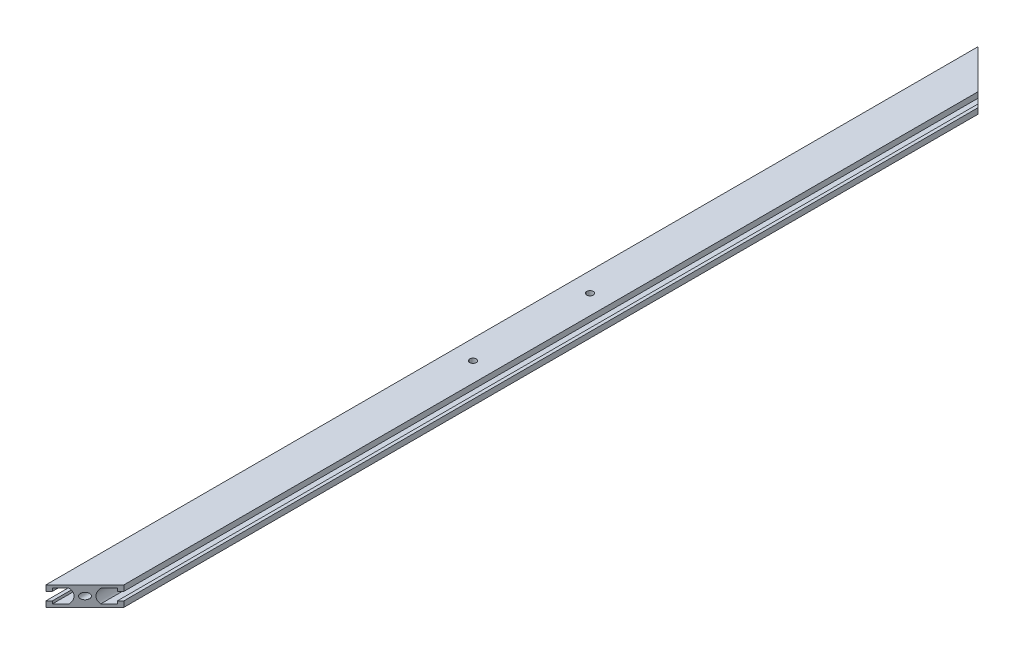
SolidWorks part; units mm, degrees
material "铝型材"
ref_plane "前视基准面" through (0, 0, 0) normal (0, 0, 1) x (1, 0, 0)
ref_plane "上视基准面" through (0, 0, 0) normal (0, 1, 0) x (1, 0, 0)
ref_plane "右视基准面" through (0, 0, 0) normal (1, 0, 0) x (0, 0, -1)
sketch "Model" plane through (0, 0, 0) normal (0, 0, 1) x (1, 0, 0)
  line L0 (2390.4271, 419.7568) -> (2392.9271, 419.7568)
  line L1 (2390.4271, 419.7568) -> (2390.4271, 417.7068)
  line L2 (2392.9271, 415.4068) -> (2392.9271, 419.7568)
  line L3 (2383.9948, 417.7068) -> (2390.4271, 417.7068)
  line L4 (2362.9271, 415.4068) -> (2392.9271, 415.4068)
  line L5 (2362.9271, 415.4068) -> (2362.9271, 419.7568)
  line L6 (2383.9948, 428.1068) -> (2390.4271, 428.1068)
  line L7 (2365.4271, 419.7568) -> (2362.9271, 419.7568)
  line L8 (2390.4271, 426.0568) -> (2390.4271, 428.1068)
  line L9 (2365.4271, 419.7568) -> (2365.4271, 417.7068)
  line L10 (2390.4271, 426.0568) -> (2392.9271, 426.0568)
  line L11 (2365.4271, 417.7068) -> (2371.8571, 417.7068)
  line L12 (2392.9271, 430.4068) -> (2392.9271, 426.0568)
  line L13 (2362.9271, 430.4068) -> (2392.9271, 430.4068)
  line L14 (2365.4271, 428.1068) -> (2371.8571, 428.1068)
  line L15 (2362.9271, 430.4068) -> (2362.9271, 426.0568)
  line L16 (2365.4271, 426.0568) -> (2365.4271, 428.1068)
  line L17 (2365.4271, 426.0568) -> (2362.9271, 426.0568)
  line L22 (2361.3714, 422.9068) -> (2394.2123, 422.9068) construction
  line L23 (2377.9271, 430.4068) -> (2377.9271, 415.4068) construction
  arc A0 (2371.8571, 428.1068) -> (2371.8571, 417.7068) centre (2365.5621, 422.9068) cw
  arc A1 (2383.9948, 428.1068) -> (2383.9948, 417.7068) centre (2390.2996, 422.9068) ccw
  circle A4 centre (2377.9271, 422.9068) radius 2.5
  point P2 (2373.7271, 422.9068)
  point P3 (2382.1271, 422.9068)
  dimension "D3" = 4.2
  dimension "D8" = 5
  dimension "D12" = 4.2
  dimension "D1" = 30
  dimension "D2" = 2.5
  dimension "D4" = 6.43
  dimension "D5" = 6.3
  dimension "D6" = 10.4
  dimension "D7" = 15
  dimension "D9" = 6.3
  dimension "D10" = 2.5
  dimension "D11" = 6.4323
extrude "凸台-拉伸1" add sketch "Model" along normal mid plane 717 contours L13 L12 L10 L8 L6 A1 L3 L1 L0 L2 L4 L5 L7 L9 L11 A0 L14 L16 L17 L15 | A4
ref_plane "基准面1" through (2382.1271, 0, 0) normal (1, 0, 0) x (0, 0, -1)
ref_plane "基准面2" through (2373.7271, 0, 0) normal (-1, 0, 0) x (0, 0, 1)
ref_plane "基准面3" through (0, 422.9068, 0) normal (0, 1, 0) x (1, 0, 0)
ref_plane "基准面4" through (2377.9271, 0, 0) normal (-1, 0, 0) x (0, 0, 1)
sketch "草图1" plane through (0, 430.4068, 0) normal (0, 1, 0) x (1, 0, 0)
  line L0 (2362.9271, 358.5) -> (2392.9271, 328.5)
  line L1 (2392.9271, -358.5) -> (2392.9271, 358.5) construction
  line L2 (2392.9271, 328.5) -> (2392.9271, 358.5)
  line L3 (2392.9271, 358.5) -> (2362.9271, 358.5)
  line L4 (2362.9271, -358.5) -> (2392.9271, -328.5)
  line L5 (2392.9271, -328.5) -> (2392.9271, -358.5)
  line L6 (2392.9271, -358.5) -> (2362.9271, -358.5)
extrude "切除-拉伸1" cut sketch "草图1" against normal through all
hole_wizard "M6 螺纹孔1" positions "草图3" profile "草图2" tap size "M6" standard "GB" end condition through all
sketch "草图3" plane through (0, 430.4068, 0) normal (0, 1, 0) x (1, 0, 0)
  point P0 (2377.9271, 45)
  point P3 (2377.9271, -45)
sketch "草图2" plane through (2377.9271, 430.4068, -45) normal (1, 0, 0) x (0, 0, 1)
  line L0 (0, 0) -> (0, 15)
  line L1 (0, 15) -> (2.5, 15)
  line L2 (2.5, 15) -> (2.5, 0)
  line L5 (2.5, 0) -> (0, 0)
  line L11 (0, -6.35) -> (0, 107.95) construction
  dimension "通孔螺纹孔钻头直径" = 5
  dimension "通孔螺纹孔钻头深度" = 15
cosmetic thread "孔螺蚊线1" parameters "D2"=6
cosmetic thread "孔螺蚊线2" parameters "D2"=6
